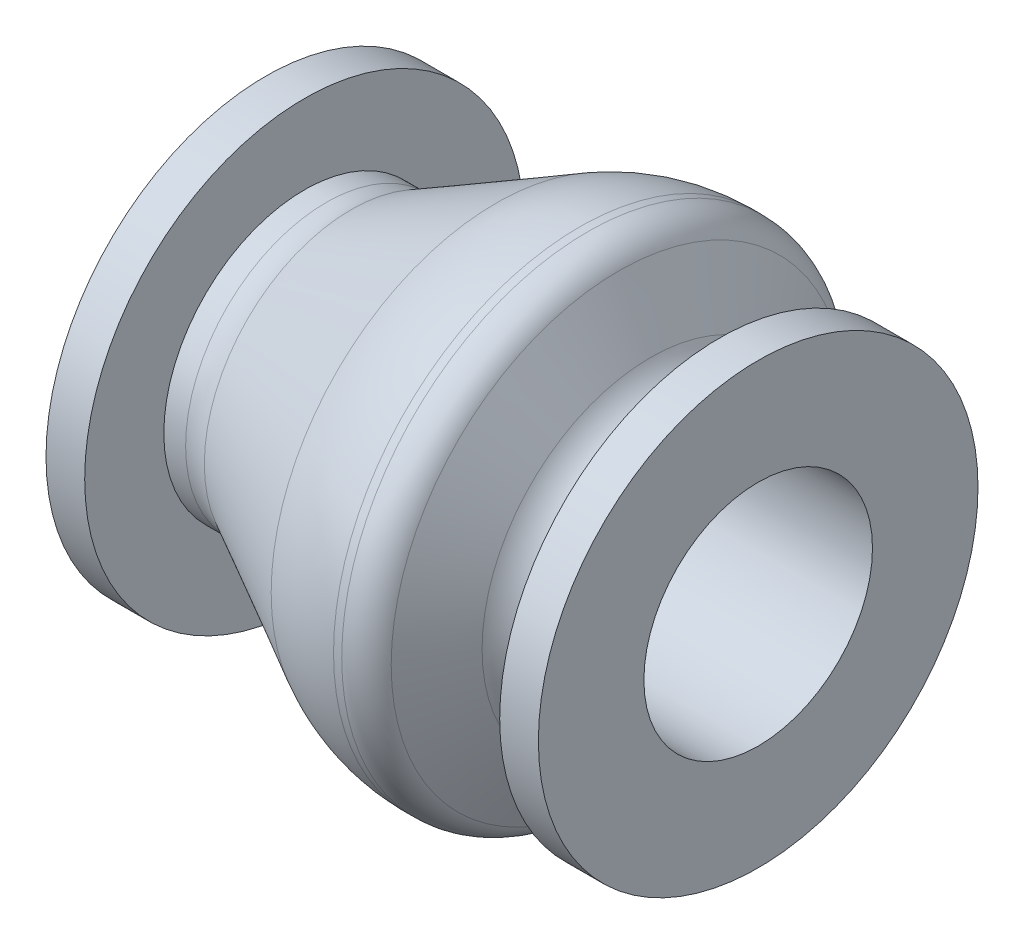
SolidWorks part; units mm, degrees
material "铸造碳钢"
ref_plane "Front Plane" through (0, 0, 0) normal (0, 0, 1) x (1, 0, 0)
ref_plane "Top Plane" through (0, 0, 0) normal (0, 1, 0) x (1, 0, 0)
ref_plane "Right Plane" through (0, 0, 0) normal (1, 0, 0) x (0, 0, -1)
sketch "Sketch1" plane through (0, 0, 0) normal (0, 0, 1) x (1, 0, 0)
  line L0 (0, 65) -> (0, 125)
  line L1 (0, 125) -> (22, 125)
  line L2 (22, 125) -> (22, 80)
  line L3 (22, 80) -> (34.3984, 80)
  line L4 (48.6214, 83.5859) -> (130.9805, 127.933)
  line L5 (178.3905, 139.8859) -> (183.0579, 139.8859)
  line L6 (200.6673, 129.3679) -> (218.7548, 95.777)
  line L7 (245.1689, 80) -> (258, 80)
  line L8 (258, 80) -> (258, 125)
  line L9 (258, 125) -> (280, 125)
  line L10 (280, 125) -> (280, 65)
  line L11 (280, 65) -> (0, 65)
  line L12 (0, 0) -> (45.6274, 0) construction
  arc A0 (218.7548, 95.777) -> (245.1689, 80) centre (245.1689, 110) ccw
  arc A1 (34.3984, 80) -> (48.6214, 83.5859) centre (34.3984, 110) ccw
  arc A2 (130.9805, 127.933) -> (178.3905, 139.8859) centre (178.3905, 39.8859) cw
  arc A3 (183.0579, 139.8859) -> (200.6673, 129.3679) centre (183.0579, 119.8859) cw
  dimension "D8" = 30
  dimension "D9" = 100
  dimension "D10" = 20
  dimension "D1" = 125
  dimension "D2" = 125
  dimension "D3" = 22
  dimension "D4" = 22
  dimension "D5" = 65
  dimension "D6" = 80
  dimension "D7" = 80
  dimension "D11" = 280
revolve "Revolve1" add sketch "Sketch1" angle 360 about L12
